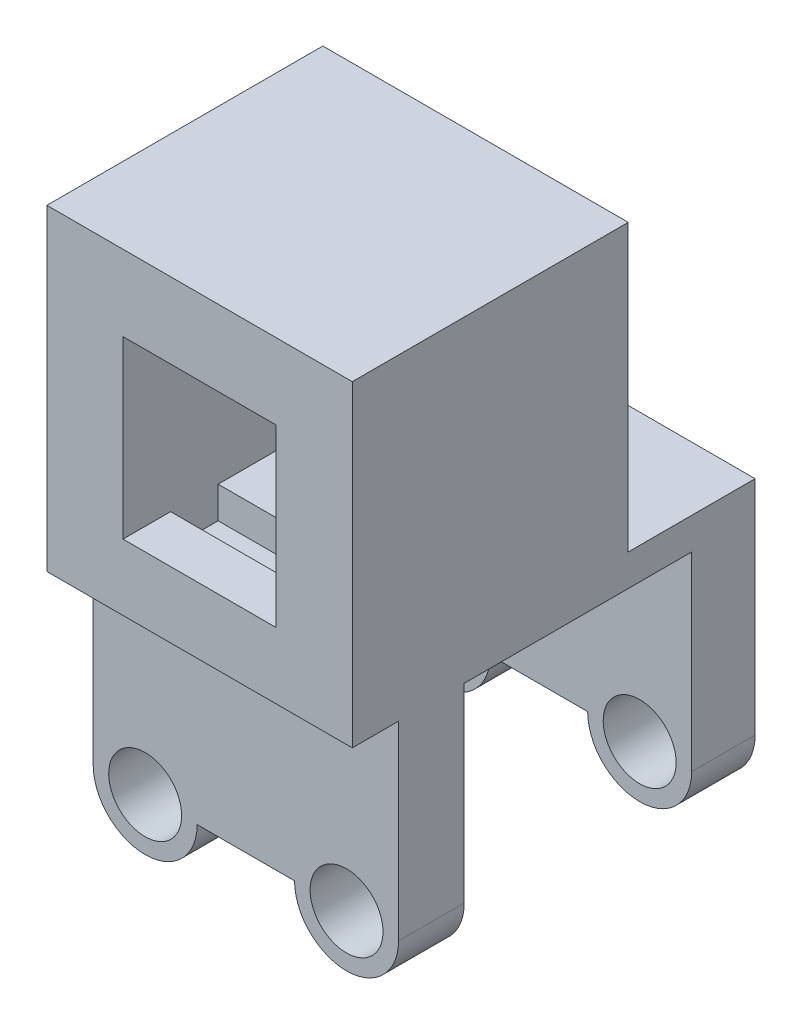
from build123d import *

# Parameters (mm, degrees)
SKETCH_1_R          = 1.64
SKETCH_1_R_2        = 1.15
EXTRUDE_1_DEPTH     = 3.1
EXTRUDE_1_2_DEPTH   = 3.1
EXTRUDE_START       = -3.1
EXTRUDE_2_DEPTH     = 3.1
SKETCH_4_W          = 9.63
SKETCH_4_H          = 10
EXTRUDE_3_DEPTH     = 5.6
SKETCH_5_W          = 4.83
SKETCH_5_H          = 5.53
CUT_EXTRUDE_1_DEPTH = 10
SKETCH_6_W          = 4.83
SKETCH_6_H          = 7.53
CUT_EXTRUDE_2_DEPTH = 1.5
SKETCH_7_W          = 2.070948157
SKETCH_7_H          = 7.64
EXTRUDE_4_DEPTH     = 9.63
SKETCH_10_R         = 1.15
CUT_EXTRUDE_3_DEPTH = 22.934678024
SKETCH_11_W         = 3.1
SKETCH_11_H         = 7.64
CUT_EXTRUDE_4_DEPTH = 21.601623722
CUT_EXTRUDE_5_DEPTH = 22.934678024


with BuildPart() as part:
    # 草图1 → 凸台-拉伸1 (new body)
    with BuildSketch(Plane.XY):
        with Locations(Location((0, 0, 0), (0, 0, 180))):
            Circle(SKETCH_1_R)
        with Locations(Location((0, 0, 0), (0, 0, 180))):
            Circle(SKETCH_1_R_2, mode=Mode.SUBTRACT)
    extrude(amount=EXTRUDE_1_DEPTH)



with BuildPart() as body_2:
    # 草图1 → Extrude 1 2 (new body)
    with BuildSketch(Plane.XY):
        with Locations(Location((-6.35, 0, 0), (0, 0, 180))):
            Circle(SKETCH_1_R)
        with Locations(Location((-6.35, 0, 0), (0, 0, 180))):
            Circle(SKETCH_1_R_2, mode=Mode.SUBTRACT)
    extrude(amount=EXTRUDE_1_2_DEPTH)


with BuildPart() as part_1:
    add(part.part)

    add(body_2.part)  # 凸台-拉伸2 merges body 2
    # 草图2 → 凸台-拉伸2 (add)
    with BuildSketch(Plane.XY.offset(3.1).offset(EXTRUDE_START)):
        with BuildLine():
            Line((-7.99, 0), (-7.99, 16))
            Line((-7.99, 16), (1.64, 16))
            Line((1.64, 16), (1.64, 0))
            ThreePointArc((1.64, 0), (0, 1.64), (-1.64, 0))
            Line((-1.64, 0), (-4.71, 0))
            ThreePointArc((-4.71, 0), (-6.35, 1.64), (-7.99, 0))
        make_face()
    extrude(amount=EXTRUDE_2_DEPTH)

    # 草图4 → 凸台-拉伸3 (add)
    with BuildSketch(Plane.XY.offset(3.1)):
        with Locations((-3.175, 11)):
            Rectangle(SKETCH_4_W, SKETCH_4_H)
    extrude(amount=EXTRUDE_3_DEPTH)

    # 草图5 → 切除-拉伸1 (cut)
    with BuildSketch(Plane.XY.offset(8.7)):
        with Locations((-3.175, 10.85)):
            Rectangle(SKETCH_5_W, SKETCH_5_H)
    extrude(amount=-CUT_EXTRUDE_1_DEPTH, mode=Mode.SUBTRACT)

    # 草图6 → 切除-拉伸2 (cut)
    with BuildSketch(Plane.XY.offset(7.2)):
        with Locations((-3.175, 10.85)):
            Rectangle(SKETCH_6_W, SKETCH_6_H)
    extrude(amount=-CUT_EXTRUDE_2_DEPTH, mode=Mode.SUBTRACT)

    # 草图7 → 凸台-拉伸4 (add)
    with BuildSketch(Plane.ZY.offset(7.99)):
        with Locations((6.206422236, 2.18)):
            Rectangle(SKETCH_7_W, SKETCH_7_H)
        Polygon((0, 6), (-2, 6), (-2, -1.64), (-4, -1.64), (-4, 6), (-4, 7), (0, 7), align=None)
    extrude(amount=-EXTRUDE_4_DEPTH)

    # 草图10 → 切除-拉伸3 (cut, through all)
    with BuildSketch(Plane(origin=(0, 0, -4), x_dir=(-1, 0, 0), z_dir=(0, 0, -1))):
        Circle(SKETCH_10_R)
        with Locations((6.35, 0)):
            Circle(SKETCH_10_R)
    extrude(amount=-CUT_EXTRUDE_3_DEPTH, mode=Mode.SUBTRACT)

    # 草图11 → 切除-拉伸4 (cut, through all)
    with BuildSketch(Plane(origin=(1.64, 0, 0), x_dir=(0, 0, -1), z_dir=(1, 0, 0))):
        with Locations((-1.55, 2.18)):
            Rectangle(SKETCH_11_W, SKETCH_11_H)
    extrude(amount=-CUT_EXTRUDE_4_DEPTH, mode=Mode.SUBTRACT)

    # 草图12 → 切除-拉伸5 (cut, through all)
    with BuildSketch(Plane(origin=(0, 0, -4), x_dir=(-1, 0, 0), z_dir=(0, 0, -1))):
        with BuildLine():
            Line((4.71, 0), (1.64, 0))
            ThreePointArc((1.64, 0), (1.159655121, -1.159655121), (0, -1.64))
            Line((0, -1.64), (6.35, -1.64))
            ThreePointArc((6.35, -1.64), (5.190344879, -1.159655121), (4.71, 0))
        make_face()
        with BuildLine():
            Line((-1.64, -1.64), (0, -1.64))
            ThreePointArc((0, -1.64), (-1.159655121, -1.159655121), (-1.64, 0))
            Line((-1.64, 0), (-1.64, -1.64))
        make_face()
        with BuildLine():
            ThreePointArc((7.99, 0), (7.509655121, -1.159655121), (6.35, -1.64))
            Line((6.35, -1.64), (7.99, -1.64))
            Line((7.99, -1.64), (7.99, 0))
        make_face()
    extrude(amount=-CUT_EXTRUDE_5_DEPTH, mode=Mode.SUBTRACT)


solid = part_1.part
